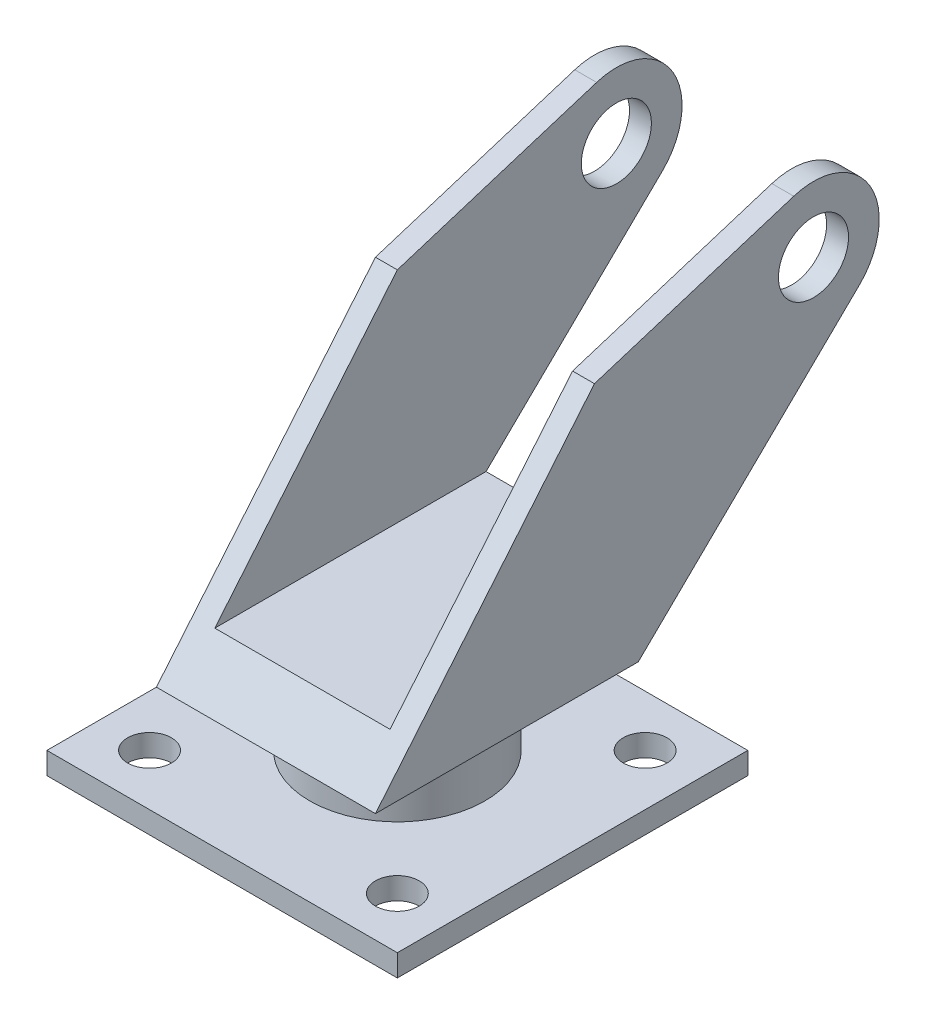
from build123d import *

# Parameters (mm, degrees)
SKETCH1_W                = 80
SKETCH1_H                = 80
SKETCH1_R                = 5
BOSS_EXTRUDE3_DEPTH      = 5
SKETCH3_R                = 20
BOSS_EXTRUDE4_DEPTH      = 15
BOSS_EXTRUDE6_DEPTH      = 25
BOSS_EXTRUDE6_DEPTH_BACK = 25
SKETCH6_R                = 8
CUT_EXTRUDE1_DEPTH       = 50
CUT_EXTRUDE1_DEPTH_BACK  = 25
SKETCH8_W                = 40
SKETCH8_H                = 200


with BuildPart() as part:
    # Sketch1 → Boss-Extrude3 (new body)
    with BuildSketch(Plane(origin=(0, 0, 0), x_dir=(1, 0, 0), z_dir=(0, 1, 0))):
        Rectangle(SKETCH1_W, SKETCH1_H)
        with Locations(Location((-28.284271247, -28.284271247, 0), (0, 0, 270))):
            Circle(SKETCH1_R, mode=Mode.SUBTRACT)
        with Locations(Location((-28.284271247, 28.284271247, 0), (0, 0, 270))):
            Circle(SKETCH1_R, mode=Mode.SUBTRACT)
        with Locations(Location((28.284271247, 28.284271247, 0), (0, 0, 270))):
            Circle(SKETCH1_R, mode=Mode.SUBTRACT)
        with Locations(Location((28.284271247, -28.284271247, 0), (0, 0, 270))):
            Circle(SKETCH1_R, mode=Mode.SUBTRACT)
    extrude(amount=BOSS_EXTRUDE3_DEPTH)

    # Sketch3 → Boss-Extrude4 (add)
    with BuildSketch(Plane(origin=(0, 5, 0), x_dir=(1, 0, 0), z_dir=(0, 1, 0))):
        with Locations(Location((0, 0, 0), (0, 0, 270))):
            Circle(SKETCH3_R)
    extrude(amount=BOSS_EXTRUDE4_DEPTH)

    # Sketch6 → Boss-Extrude6 (add, two sides: drawn at the far end of the back side and taken through both)
    with BuildSketch(Plane(origin=(0, 0, 0), x_dir=(0, 0, -1), z_dir=(1, 0, 0)).offset(-BOSS_EXTRUDE6_DEPTH_BACK)):
        with BuildLine():
            Line((0, 20), (30, 20))
            Line((30, 20), (80.476983059, 69.265344627))
            ThreePointArc((80.476983059, 69.265344627), (82.87355244, 87.698808192), (65.5, 94.309088021))
            Line((65.5, 94.309088021), (20, 80))
            Line((20, 80), (-30, 20))
            Line((-30, 20), (0, 20))
        make_face()
        with Locations((70, 80)):
            Circle(SKETCH6_R, mode=Mode.SUBTRACT)
    extrude(amount=BOSS_EXTRUDE6_DEPTH + BOSS_EXTRUDE6_DEPTH_BACK)

    # Sketch8 → Cut-Extrude1 (cut, two sides: drawn at the far end of the back side and taken through both)
    with BuildSketch(Plane(origin=(0, 80, 0), x_dir=(-1, 0, 0), z_dir=(0, -1, 0)).offset(-CUT_EXTRUDE1_DEPTH_BACK)):
        Rectangle(SKETCH8_W, SKETCH8_H)
    extrude(amount=CUT_EXTRUDE1_DEPTH + CUT_EXTRUDE1_DEPTH_BACK, mode=Mode.SUBTRACT)


solid = part.part
